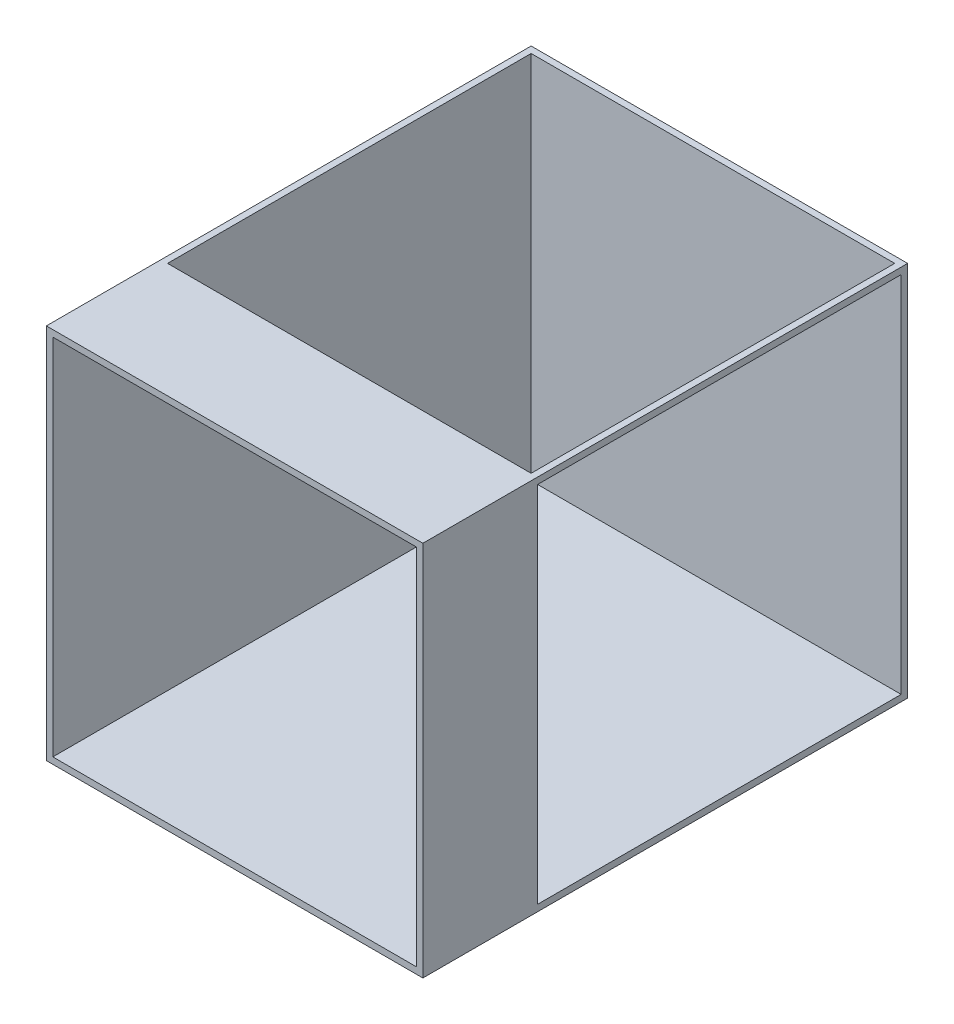
SolidWorks part; units mm, degrees
ref_plane "Front Plane" through (0, 0, 0) normal (0, 0, 1) x (1, 0, 0)
ref_plane "Top Plane" through (0, 0, 0) normal (0, 1, 0) x (1, 0, 0)
ref_plane "Right Plane" through (0, 0, 0) normal (1, 0, 0) x (0, 0, -1)
other "Configuration Table"
sketch "Sketch2" plane through (0, 0, 0) normal (0, 0, 1) x (1, 0, 0)
  line L1 (-225, 225) -> (225, 225)
  line L2 (-225, 225) -> (-225, -225)
  line L3 (-225, -225) -> (225, -225)
  line L4 (225, 225) -> (225, -225)
  line L5 (-225, 225) -> (225, -225) construction
  line L6 (-225, -225) -> (225, 225) construction
  line L7 (-233, 233) -> (233, 233)
  line L8 (-233, 233) -> (-233, -233)
  line L9 (-233, -233) -> (233, -233)
  line L10 (233, 233) -> (233, -233)
  line L11 (-233, 233) -> (233, -233) construction
  line L12 (-233, -233) -> (233, 233) construction
  point P0 (0, 0)
  point P6 (0, 0)
  dimension "D1" = 450
  dimension "D2" = 450
  dimension "D3" = 466
  dimension "D4" = 466
extrude "Boss-Extrude1" add sketch "Sketch2" along normal mid plane 600
sketch "Sketch4" plane through (-225, 0, 0) normal (1, 0, 0) x (0, 0, -1)
  line L0 (-300, 233) -> (300, 233) construction
  line L1 (300, 233) -> (292, 233)
  line L2 (300, 233) -> (300, -233)
  line L3 (300, -233) -> (292, -233)
  line L4 (292, 233) -> (292, -233)
  line L5 (300, -233) -> (300, 233) construction
  line L6 (-300, -233) -> (300, -233) construction
  dimension "D1" = 8
extrude "Boss-Extrude2" add sketch "Sketch4" along normal blind 450
sketch "Sketch5" plane through (0, 233, 0) normal (0, 1, 0) x (1, 0, 0)
  line L0 (233, 300) -> (-233, 300) construction
  line L1 (-225, 292) -> (225, 292)
  line L2 (-225, 292) -> (-225, -158)
  line L3 (-225, -158) -> (225, -158)
  line L4 (225, 292) -> (225, -158)
  line L5 (233, -300) -> (233, 300) construction
  line L6 (-233, -300) -> (-233, 300) construction
  dimension "D1" = 8
  dimension "D2" = 8
  dimension "D3" = 8
  dimension "D4" = 450
extrude "Cut-Extrude1" cut sketch "Sketch5" against normal blind 8
sketch "Sketch6" plane through (233, 0, 0) normal (1, 0, 0) x (0, 0, -1)
  line L0 (300, -233) -> (300, 233) construction
  line L1 (292, 225) -> (-158, 225)
  line L2 (292, 225) -> (292, -225)
  line L3 (292, -225) -> (-158, -225)
  line L4 (-158, 225) -> (-158, -225)
  line L5 (-300, 233) -> (300, 233) construction
  line L6 (-300, -233) -> (300, -233) construction
  dimension "D1" = 8
  dimension "D2" = 8
  dimension "D3" = 8
  dimension "D4" = 450
extrude "Cut-Extrude2" cut sketch "Sketch6" against normal blind 8
